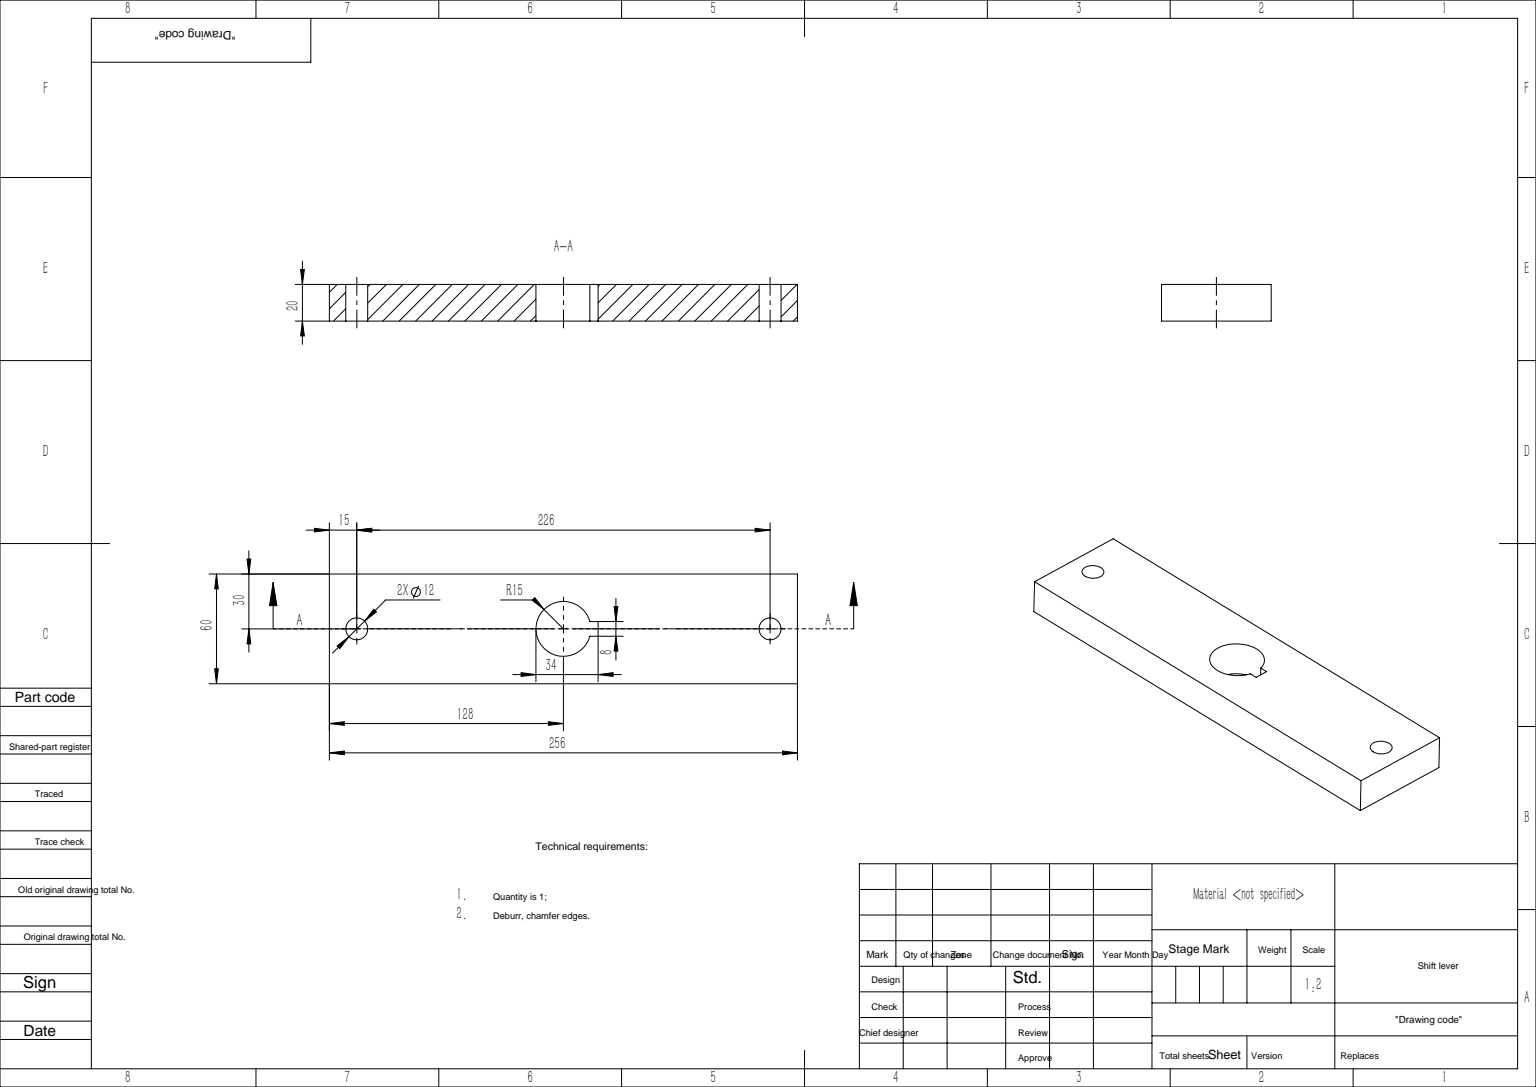
SolidWorks part; units mm, degrees
ref_plane "前视基准面" through (0, 0, 0) normal (0, 0, 1) x (1, 0, 0)
ref_plane "上视基准面" through (0, 0, 0) normal (0, 1, 0) x (1, 0, 0)
ref_plane "右视基准面" through (0, 0, 0) normal (1, 0, 0) x (0, 0, -1)
sketch "草图1" plane through (0, 0, 0) normal (0, 0, 1) x (1, 0, 0)
  line L1 (-30, -128) -> (30, -128)
  line L2 (-30, -128) -> (-30, 128)
  line L3 (-30, 128) -> (30, 128)
  line L4 (30, -128) -> (30, 128)
  line L5 (-30, -128) -> (30, 128) construction
  line L6 (-30, 128) -> (30, -128) construction
  point P0 (0, 0)
  dimension "D1" = 256
  dimension "D2" = 60
extrude "凸台-拉伸1" add sketch "草图1" along normal blind 20
sketch "草图2" plane through (0, 0, 20) normal (0, 0, 1) x (1, 0, 0)
  line L0 (0, 0) -> (80, 0) construction
  line L1 (0, 0) -> (0, 200) construction
  circle A0 centre (0, 113) radius 6
  circle A1 centre (0, -113) radius 6
  dimension "D1" = 12
  dimension "D2" = 200
  dimension "D3" = 80
  dimension "D4" = 226
extrude "切除-拉伸1" cut sketch "草图2" against normal through all
sketch "草图3" plane through (0, 0, 20) normal (0, 0, 1) x (1, 0, 0)
  line L0 (0, 0) -> (0, 40) construction
  line L1 (-4, 19) -> (4, 19)
  line L2 (-4, 19) -> (-4, 14.4568)
  line L4 (4, 19) -> (4, 14.4568)
  arc A0 (-4, 14.4568) -> (4, 14.4568) centre (0, 0) ccw
  dimension "D1" = 40
  dimension "D3" = 30
  dimension "D2" = 19
  dimension "D4" = 8
extrude "切除-拉伸2" cut sketch "草图3" against normal through all
